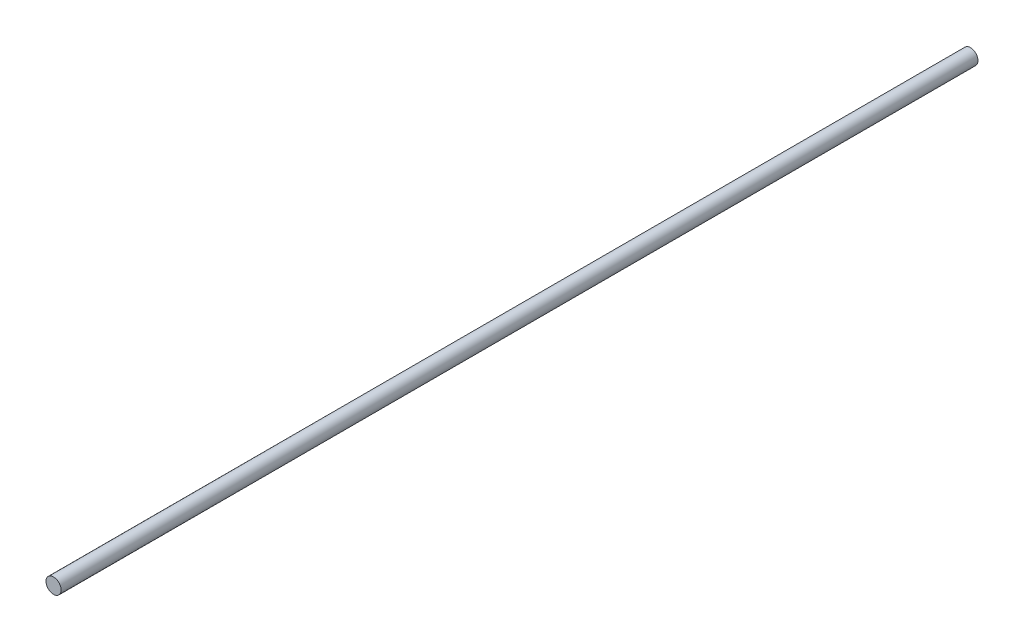
SolidWorks part; units mm, degrees
ref_plane "前视基准面" through (0, 0, 0) normal (0, 0, 1) x (1, 0, 0)
ref_plane "上视基准面" through (0, 0, 0) normal (0, 1, 0) x (1, 0, 0)
ref_plane "右视基准面" through (0, 0, 0) normal (1, 0, 0) x (0, 0, -1)
other "Configuration Table"
sketch "草图1" plane through (0, 0, 0) normal (0, 0, 1) x (1, 0, 0)
  circle A0 centre (0, 0) radius 8
  point P0 (0, 0)
  dimension "D1" = 16
extrude "凸台-拉伸1" add sketch "草图1" against normal mid plane 970
